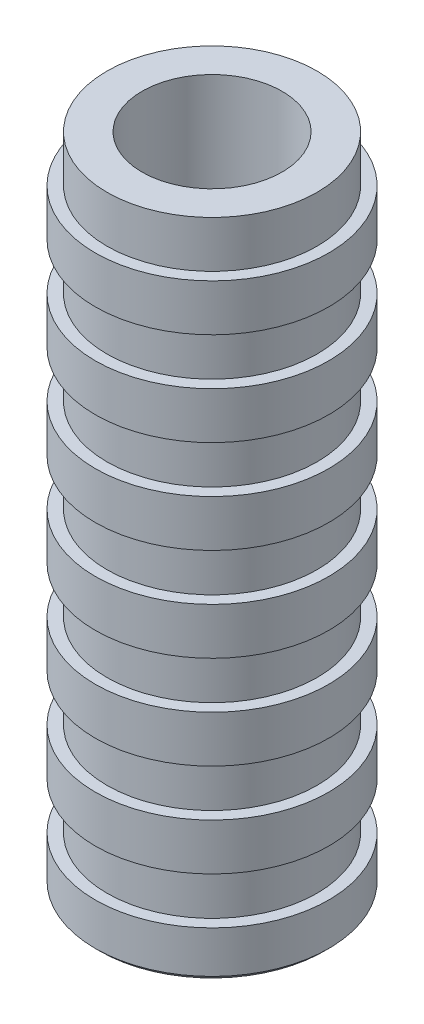
SolidWorks part; units mm, degrees
ref_plane "前视基准面" through (0, 0, 0) normal (0, 0, 1) x (1, 0, 0)
ref_plane "上视基准面" through (0, 0, 0) normal (0, 1, 0) x (1, 0, 0)
ref_plane "右视基准面" through (0, 0, 0) normal (1, 0, 0) x (0, 0, -1)
ref_plane "基准面4" through (0, 0, 0) normal (0, 0, -1) x (-1, 0, 0)
sketch "草图1" plane through (0, 0, 0) normal (0, 0, -1) x (-1, 0, 0)
  line L0 (-22.5, -220) -> (-25, -220)
  line L1 (-25, -220) -> (-25, -230)
  line L2 (-25, -230) -> (-22.5, -230)
  line L3 (-22.5, -230) -> (-22.5, -240)
  line L4 (-22.5, -240) -> (-25, -240)
  line L5 (-25, -240) -> (-25, -250)
  line L6 (-25, -250) -> (-22.5, -250)
  line L7 (-22.5, -250) -> (-22.5, -260)
  line L8 (-22.5, -260) -> (-25, -260)
  line L9 (-25, -260) -> (-25, -270)
  line L10 (-25, -270) -> (-22.5, -270)
  line L11 (-22.5, -270) -> (-22.5, -280)
  line L12 (-22.5, -280) -> (-25, -280)
  line L13 (-25, -280) -> (-25, -289)
  line L14 (-25, -289) -> (-24, -290)
  line L15 (-24, -290) -> (-16, -290)
  line L16 (-16, -290) -> (-15, -289)
  line L17 (-15, -289) -> (-15, -150)
  line L18 (-15, -150) -> (-22.5, -150)
  line L19 (-22.5, -150) -> (-22.5, -160)
  line L20 (-22.5, -160) -> (-25, -160)
  line L21 (-25, -160) -> (-25, -170)
  line L22 (-25, -170) -> (-22.5, -170)
  line L23 (-22.5, -170) -> (-22.5, -180)
  line L24 (-22.5, -180) -> (-25, -180)
  line L25 (-25, -180) -> (-25, -190)
  line L26 (-25, -190) -> (-22.5, -190)
  line L27 (-22.5, -190) -> (-22.5, -200)
  line L28 (-22.5, -200) -> (-25, -200)
  line L29 (-25, -200) -> (-25, -210)
  line L30 (-25, -210) -> (-22.5, -210)
  line L31 (-22.5, -210) -> (-22.5, -220)
  line L32 (0, -290) -> (0, -150) construction
revolve "旋转1" add sketch "草图1" angle 360 about L32
